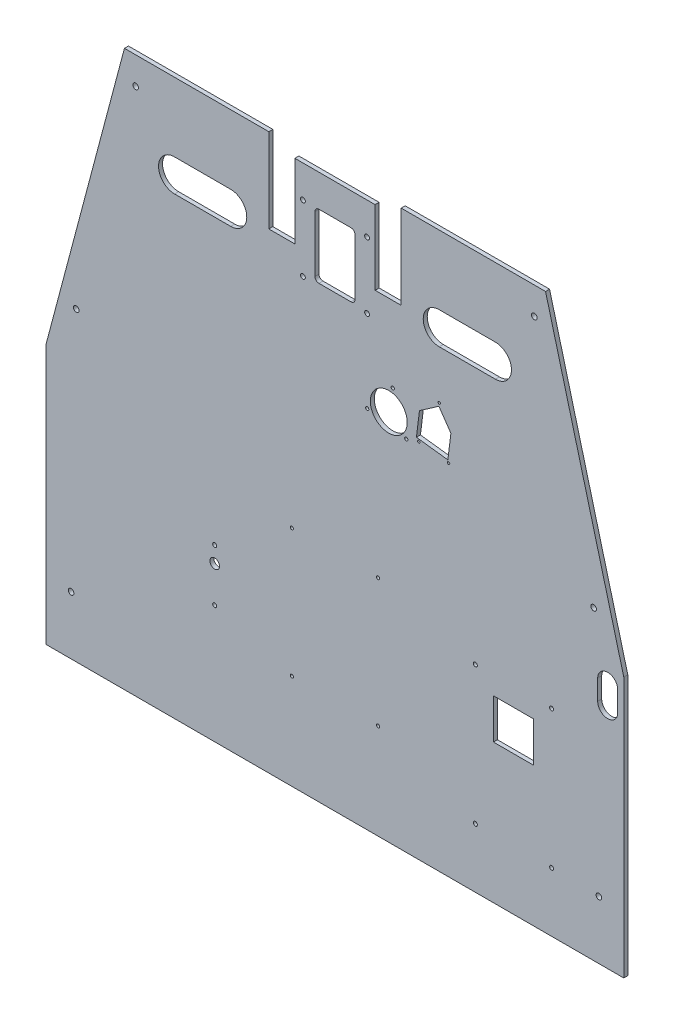
SolidWorks part; units mm, degrees
material "Plain Carbon Steel"
ref_plane "Front Plane" through (0, 0, 0) normal (0, 0, 1) x (1, 0, 0)
ref_plane "Top Plane" through (0, 0, 0) normal (0, 1, 0) x (1, 0, 0)
ref_plane "Right Plane" through (0, 0, 0) normal (1, 0, 0) x (0, 0, -1)
sketch "Sketch1" plane through (0, 0, 0) normal (0, 0, 1) x (1, 0, 0)
  line L0 (0, -12743.2508) -> (0, 624419.2913) construction
  line L1 (-12743.2508, 0) -> (624419.2913, 0) construction
  line L2 (-720, 0) -> (720, 0)
  line L3 (720, 0) -> (720, 650)
  line L4 (720, 650) -> (525, 1385)
  line L5 (525, 1385) -> (-525, 1385)
  line L6 (-525, 1385) -> (-720, 650)
  line L7 (-720, 650) -> (-720, 0)
  dimension "D1" = 1440
  dimension "D2" = 650
  dimension "D3" = 1385
  dimension "D4" = 1050
extrude "Boss-Extrude1" add sketch "Sketch1" along normal blind 10
sketch "Sketch2" plane through (0, 0, 10) normal (0, 0, 1) x (1, 0, 0)
  line L0 (-720, 0) -> (720, 0) construction
  circle A0 centre (-658, 145) radius 7
  dimension "D1" = 14
  dimension "D2" = 145
  dimension "D3" = 658
extrude "Cut-Extrude1" cut sketch "Sketch2" against normal blind 10
pattern_linear "LPattern1" count 2 spacing 1316 along (1, 0, 0) of "Cut-Extrude1"
sketch "Sketch3" plane through (0, 0, 10) normal (0, 0, 1) x (1, 0, 0)
  line L0 (-720, 0) -> (720, 0) construction
  circle A0 centre (-645, 762) radius 7
  dimension "D1" = 14
  dimension "D2" = 762
  dimension "D3" = 645
extrude "Cut-Extrude2" cut sketch "Sketch3" against normal blind 10
pattern_linear "LPattern2" count 2 spacing 1290 along (1, 0, 0) of "Cut-Extrude2"
sketch "Sketch4" plane through (0, 0, 10) normal (0, 0, 1) x (1, 0, 0)
  line L0 (-720, 0) -> (720, 0) construction
  circle A0 centre (-497, 1317) radius 7
  dimension "D1" = 14
  dimension "D2" = 1317
  dimension "D3" = 497
extrude "Cut-Extrude3" cut sketch "Sketch4" against normal blind 10
pattern_linear "LPattern3" count 2 spacing 994 along (1, 0, 0) of "Cut-Extrude3"
sketch "Sketch5" plane through (0, 0, 10) normal (0, 0, 1) x (1, 0, 0)
  line L0 (-720, 0) -> (720, 0) construction
  line L1 (720, 0) -> (720, 650) construction
  line L2 (655, 615) -> (655, 565)
  line L3 (705, 615) -> (705, 565)
  arc A0 (655, 565) -> (705, 565) centre (680, 565) ccw
  arc A1 (705, 615) -> (655, 615) centre (680, 615) ccw
  dimension "D4" = 25
  dimension "D1" = 565
  dimension "D2" = 50
  dimension "D3" = 40
extrude "Cut-Extrude4" cut sketch "Sketch5" against normal blind 10
sketch "Sketch6" plane through (0, 0, 10) normal (0, 0, 1) x (1, 0, 0)
  line L0 (720, 0) -> (720, 650) construction
  line L1 (395, 447) -> (495, 447)
  line L2 (395, 447) -> (395, 347)
  line L3 (395, 347) -> (495, 347)
  line L4 (495, 447) -> (495, 347)
  line L5 (-720, 0) -> (720, 0) construction
  dimension "D1" = 225
  dimension "D2" = 347
  dimension "D3" = 100
  dimension "D4" = 100
extrude "Cut-Extrude5" cut sketch "Sketch6" against normal blind 10
sketch "Sketch7" plane through (0, 0, 10) normal (0, 0, 1) x (1, 0, 0)
  line L0 (720, 0) -> (720, 650) construction
  line L1 (-720, 0) -> (720, 0) construction
  circle A0 centre (540, 492) radius 5
  dimension "D1" = 10
  dimension "D2" = 180
  dimension "D3" = 492
extrude "Cut-Extrude6" cut sketch "Sketch7" against normal blind 10
pattern_linear "LPattern4" count 2 spacing 190 along (-1, 0, 0) count 2 spacing 344 along (0, -1, 0) of "Cut-Extrude6"
sketch "Sketch8" plane through (0, 0, 10) normal (0, 0, 1) x (1, 0, 0)
  line L0 (-720, 0) -> (720, 0) construction
  circle A0 centre (107.5, 238) radius 4
  dimension "D1" = 8
  dimension "D2" = 107.5
  dimension "D3" = 238
extrude "Cut-Extrude7" cut sketch "Sketch8" against normal blind 10
pattern_linear "LPattern5" count 2 spacing 320 along (0, 1, 0) count 2 spacing 215 along (-1, 0, 0) of "Cut-Extrude7"
sketch "Sketch9" plane through (0, 0, 10) normal (0, 0, 1) x (1, 0, 0)
  line L0 (-400, 1133) -> (-260, 1133)
  line L1 (-260, 1213) -> (-400, 1213)
  line L3 (525, 1385) -> (-525, 1385) construction
  arc A0 (-260, 1133) -> (-260, 1213) centre (-260, 1173) ccw
  arc A1 (-400, 1213) -> (-400, 1133) centre (-400, 1173) ccw
  dimension "D3" = 260
  dimension "D1" = 80
  dimension "D2" = 80
  dimension "D4" = 212
  dimension "D5" = 140
extrude "Cut-Extrude8" cut sketch "Sketch9" against normal blind 10
pattern_linear "LPattern6" count 2 spacing 660 along (1, 0, 0) of "Cut-Extrude8"
sketch "Sketch10" plane through (0, 0, 10) normal (0, 0, 1) x (1, 0, 0)
  line L0 (0, -1000) -> (0, 49000) construction
  line L1 (525, 1385) -> (-525, 1385) construction
  line L2 (-50, 1280) -> (50, 1280)
  line L3 (-50, 1280) -> (-50, 1120)
  line L4 (-50, 1120) -> (50, 1120)
  line L5 (50, 1280) -> (50, 1120)
  dimension "D1" = 105
  dimension "D2" = 160
  dimension "D3" = 100
extrude "Cut-Extrude9" cut sketch "Sketch10" against normal blind 10
fillet "Fillet1" radius 10 4 edges at (50, 1120, 5) (-50, 1120, 5) (50, 1280, 5) (-50, 1280, 5)
sketch "Sketch11" plane through (0, 0, 10) normal (0, 0, 1) x (1, 0, 0)
  line L0 (525, 1385) -> (-525, 1385) construction
  circle A0 centre (80, 1280) radius 6
  dimension "D1" = 12
  dimension "D2" = 80
  dimension "D3" = 105
extrude "Cut-Extrude10" cut sketch "Sketch11" against normal blind 10
pattern_linear "LPattern7" count 2 spacing 160 along (-1, 0, 0) count 2 spacing 165 along (0, -1, 0) of "Cut-Extrude10"
sketch "Sketch12" plane through (0, 0, 10) normal (0, 0, 1) x (1, 0, 0)
  line L0 (525, 1385) -> (-525, 1385) construction
  circle A0 centre (144, 986) radius 4
  dimension "D1" = 8
  dimension "D2" = 399
  dimension "D3" = 144
extrude "Cut-Extrude11" cut sketch "Sketch12" against normal blind 10
sketch "Sketch14" plane through (0, 0, 10) normal (0, 0, 1) x (1, 0, 0)
  line L0 (0, -1000) -> (0, 49000) construction
  line L1 (144, 986) -> (-8538.4089, -48254.3877) construction
  circle A0 centre (134.0673, 929.669) radius 46
  point P6 (144, 986)
  dimension "D3" = 92
  dimension "D1" = 10
  dimension "D2" = 57.2
extrude "Cut-Extrude12" cut sketch "Sketch14" against normal blind 10
sketch "Sketch15" plane through (0, 0, 10) normal (0, 0, 1) x (1, 0, 0)
  line L0 (144, 986) -> (129.0663, 901.3065) construction
  line L1 (36.8819, 917.5611) -> (204.7665, 887.9585) construction
  line L2 (0, -1000) -> (0, 49000) construction
  circle A0 centre (80.3183, 909.9021) radius 4
  dimension "D3" = 8
  dimension "D1" = 90
  dimension "D2" = 86
  dimension "D4" = 49.5
  dimension "D5" = 10
extrude "Cut-Extrude13" cut sketch "Sketch15" against normal blind 10
pattern_linear "LPattern8" count 2 spacing 99 along (0.9848, -0.1736, 0) of "Cut-Extrude13"
sketch "Sketch16" plane through (0, 0, 10) normal (0, 0, 1) x (1, 0, 0)
  line L0 (525, 1385) -> (-525, 1385) construction
  circle A0 centre (260, 1012) radius 3
  dimension "D3" = 6
  dimension "D1" = 260
  dimension "D2" = 373
extrude "Cut-Extrude14" cut sketch "Sketch16" against normal blind 10
sketch "Sketch17" plane through (0, 0, 10) normal (0, 0, 1) x (1, 0, 0)
  line L0 (0, -1000) -> (0, 49000) construction
  line L1 (260, 1012) -> (-5833.4672, -48615.3076) construction
  line L2 (259.025, 1004.0596) -> (210.5705, 970.4716)
  line L3 (259.025, 1004.0596) -> (288.9817, 960.8439)
  line L4 (210.5705, 970.4716) -> (203.0442, 909.1747)
  line L5 (288.9817, 960.8439) -> (281.4554, 899.547)
  line L6 (281.4554, 899.547) -> (203.0442, 909.1747)
  point P6 (260, 1012)
  dimension "D1" = 7
  dimension "D2" = 109
  dimension "D3" = 79
  dimension "D4" = 44
  dimension "D5" = 8
extrude "Cut-Extrude15" cut sketch "Sketch17" against normal blind 10
sketch "Sketch18" plane through (0, 0, 10) normal (0, 0, 1) x (1, 0, 0)
  line L0 (0, -1000) -> (0, 49000) construction
  line L1 (260, 1012) -> (-5833.4672, -48615.3076) construction
  line L2 (208.7645, 902.4273) -> (280.1734, 893.6594) construction
  circle A0 centre (208.7645, 902.4273) radius 3
  circle A2 centre (260, 1012) radius 3 construction
  dimension "D2" = 6
  dimension "D1" = 7
  dimension "D3" = 37.5
  dimension "D4" = 90
  dimension "D5" = 115
extrude "Cut-Extrude16" cut sketch "Sketch18" against normal blind 10
pattern_linear "LPattern9" count 2 spacing 75 along (0.9925, -0.1219, 0) of "Cut-Extrude16"
sketch "Sketch19" plane through (0, 0, 10) normal (0, 0, 1) x (1, 0, 0)
  line L0 (-720, 0) -> (720, 0) construction
  circle A0 centre (-300, 295) radius 5
  dimension "D3" = 10
  dimension "D1" = 300
  dimension "D2" = 295
extrude "Cut-Extrude17" cut sketch "Sketch19" against normal blind 10
pattern_linear "LPattern10" count 2 spacing 130 along (0, 1, 0) of "Cut-Extrude17"
sketch "Sketch20" plane through (0, 0, 10) normal (0, 0, 1) x (1, 0, 0)
  line L0 (-720, 0) -> (720, 0) construction
  circle A0 centre (-300, 385) radius 12
  dimension "D3" = 24
  dimension "D1" = 300
  dimension "D2" = 385
extrude "Cut-Extrude18" cut sketch "Sketch20" against normal blind 10
ref_plane "Plane2" through (0, 0, 0) normal (1, 0, 0) x (0, 0, -1)
sketch "Sketch21" plane through (0, 0, 10) normal (0, 0, 1) x (1, 0, 0)
  line L0 (525, 1385) -> (-525, 1385) construction
  line L1 (100, 1385) -> (165, 1385)
  line L2 (100, 1385) -> (100, 1175)
  line L3 (100, 1175) -> (165, 1175)
  line L4 (165, 1385) -> (165, 1175)
  line L5 (0, -5.5) -> (0, 5.5) construction
  dimension "D1" = 210
  dimension "D2" = 100
  dimension "D3" = 165
extrude "Cut-Extrude19" cut sketch "Sketch21" against normal blind 10
sketch "Sketch22" plane through (0, 0, 10) normal (0, 0, 1) x (1, 0, 0)
  line L0 (100, 1385) -> (-525, 1385) construction
  line L1 (-165, 1385) -> (-100, 1385)
  line L2 (-165, 1385) -> (-165, 1175)
  line L3 (-165, 1175) -> (-100, 1175)
  line L4 (-100, 1385) -> (-100, 1175)
  line L5 (0, -5.5) -> (0, 5.5) construction
  dimension "D1" = 210
  dimension "D2" = 100
  dimension "D3" = 165
extrude "Cut-Extrude20" cut sketch "Sketch22" against normal blind 10
sketch "Sketch23" plane through (0, 0, 10) normal (0, 0, 1) x (1, 0, 0)
  line L0 (100, 1385) -> (100, 1175) construction
  line L1 (-100, 1385) -> (100, 1385)
  line L2 (-100, 1385) -> (-100, 1360)
  line L3 (-100, 1360) -> (100, 1360)
  line L4 (100, 1385) -> (100, 1360)
  line L5 (100, 1175) -> (165, 1175) construction
  point P7 (132.5, 1175)
  dimension "D1" = 185
extrude "Cut-Extrude21" cut sketch "Sketch23" against normal blind 10
